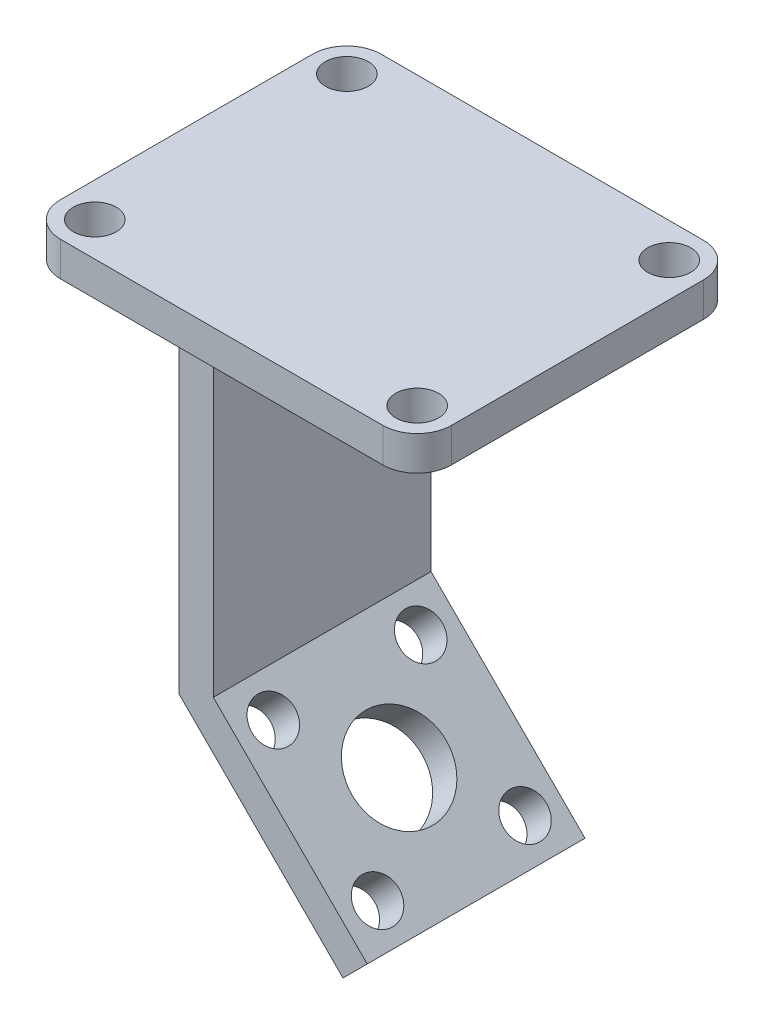
from build123d import *

# Parameters (mm, degrees)
EXTRUDE_THIN1_DEPTH     = 12.7
SKETCH3_W               = 22.8
SKETCH3_H               = 18.7
BOSS_EXTRUDE2_DEPTH     = 2
FILLET1_R               = 2
SKETCH4_R               = 1.25
CUT_EXTRUDE1_DEPTH      = 2
CUT_EXTRUDE2_DEPTH      = 61.42253709
CUT_EXTRUDE2_DEPTH_BACK = 61.42253709
SKETCH5_R               = 2.75
SKETCH6_R               = 1.25
CUT_EXTRUDE3_DEPTH      = 10


with BuildPart() as part:
    # Sketch1 → Extrude-Thin1 (new body)
    with BuildSketch(Plane.XY):
        Polygon((51.165574182, 84.975681723), (42.185318061, 93.955937844), (42.185318061, 113.634045339), (40.185318061, 113.634045339), (40.185318061, 93.127510719), (49.75136062, 83.561468161), align=None)
    extrude(amount=-EXTRUDE_THIN1_DEPTH)

    # Sketch5 → Cut-Extrude2 (cut, two sides: drawn at the far end of the back side and taken through both)
    with BuildSketch(Plane(origin=(68.070627953, 68.070627953, 0), x_dir=(0, 0, -1), z_dir=(0.7071067811865513, 0.7071067811865437, 0)).offset(-CUT_EXTRUDE2_DEPTH_BACK)):
        with Locations(Location((6.35, 30.257356315, 0), (0, 0, 90))):
            Circle(SKETCH5_R)
    extrude(amount=CUT_EXTRUDE2_DEPTH + CUT_EXTRUDE2_DEPTH_BACK, mode=Mode.SUBTRACT)

    # Sketch6 → Cut-Extrude3 (cut)
    with BuildSketch(Plane(origin=(66.65641439, 66.65641439, 0), x_dir=(0, 0, 1), z_dir=(-0.7071067811865513, -0.7071067811865437, 0))):
        with Locations(Location((-10.65, 34.557356315, 0), (0, 0, 270))):
            Circle(SKETCH6_R)
        with Locations(Location((-2.05, 34.557356315, 0), (0, 0, 270))):
            Circle(SKETCH6_R)
        with Locations(Location((-2.05, 25.957356315, 0), (0, 0, 270))):
            Circle(SKETCH6_R)
        with Locations(Location((-10.65, 25.957356315, 0), (0, 0, 270))):
            Circle(SKETCH6_R)
    extrude(amount=-CUT_EXTRUDE3_DEPTH, mode=Mode.SUBTRACT)


with BuildPart() as body_2:
    # Sketch3 → Boss-Extrude2 (new body)
    with BuildSketch(Plane(origin=(0, 113.634045339, 0), x_dir=(1, 0, 0), z_dir=(0, 1, 0))):
        with Locations((45.675446122, 6.35)):
            Rectangle(SKETCH3_W, SKETCH3_H)
    extrude(amount=BOSS_EXTRUDE2_DEPTH)

    # Fillet1
    fillet1_edges = [body_2.edges().sort_by_distance(p)[0] for p in [
        (57.075446122, 114.634045339, 3),
        (34.275446122, 114.634045339, 3),
        (34.275446122, 114.634045339, -15.7),
        (57.075446122, 114.634045339, -15.7),
    ]]
    fillet(fillet1_edges, radius=FILLET1_R)

    # Sketch4 → Cut-Extrude1 (cut)
    with BuildSketch(Plane(origin=(0, 115.634045339, 0), x_dir=(1, 0, 0), z_dir=(0, 1, 0))):
        with Locations(Location((55.075446122, 13.7, 0), (0, 0, 270))):
            Circle(SKETCH4_R)
        with Locations(Location((55.075446122, -1, 0), (0, 0, 270))):
            Circle(SKETCH4_R)
        with Locations(Location((36.275446122, -1, 0), (0, 0, 270))):
            Circle(SKETCH4_R)
        with Locations(Location((36.275446122, 13.7, 0), (0, 0, 270))):
            Circle(SKETCH4_R)
    extrude(amount=-CUT_EXTRUDE1_DEPTH, mode=Mode.SUBTRACT)


solid = Compound([part.part, body_2.part])
